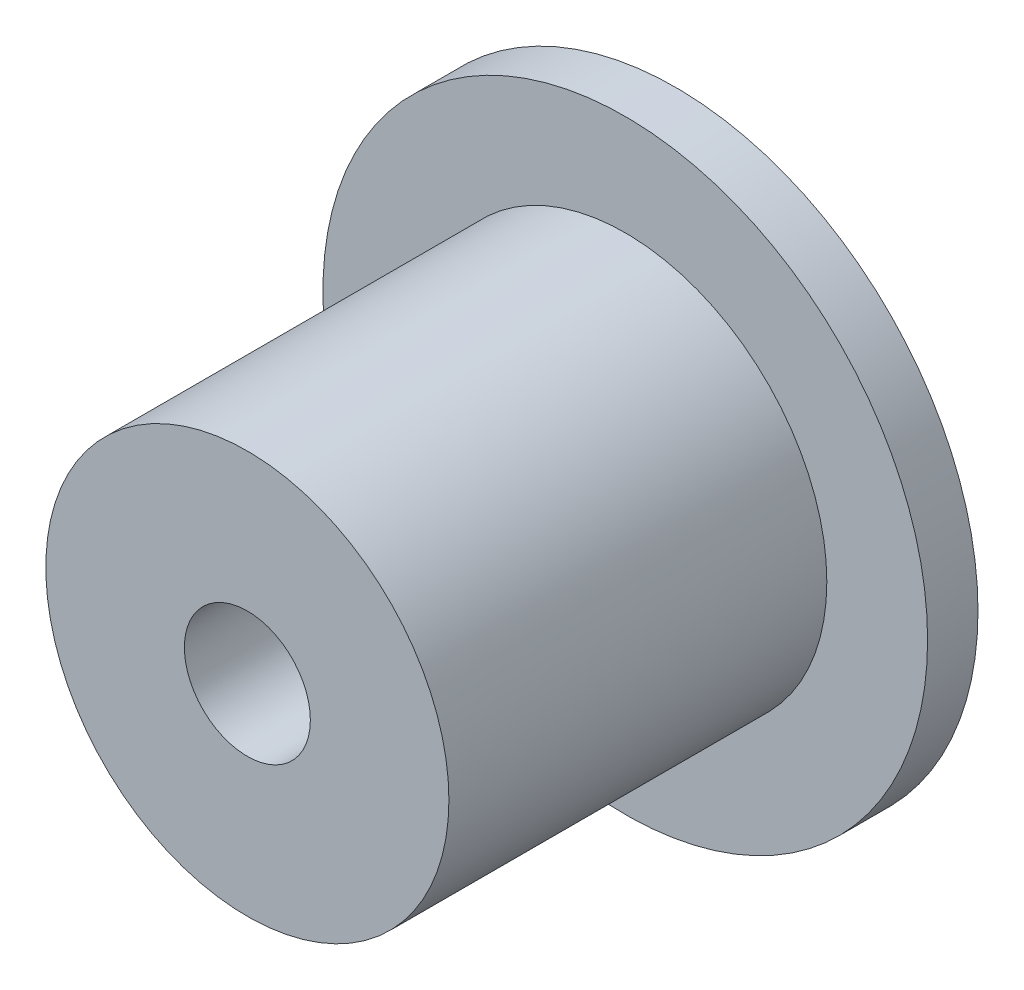
SolidWorks part; units mm, degrees
ref_plane "前视基准面" through (0, 0, 0) normal (0, 0, 1) x (1, 0, 0)
ref_plane "上视基准面" through (0, 0, 0) normal (0, 1, 0) x (1, 0, 0)
ref_plane "右视基准面" through (0, 0, 0) normal (1, 0, 0) x (0, 0, -1)
other "Configuration Table"
sketch "草图1" plane through (0, 0, 0) normal (0, 0, 1) x (1, 0, 0)
  circle A0 centre (0, 0) radius 4
  circle A1 centre (0, 0) radius 1.25
  point P0 (0, 0)
  dimension "D1" = 2.5
  dimension "D2" = 8
extrude "凸台-拉伸1" add sketch "草图1" along normal blind 7.5
sketch "草图2" plane through (0, 0, 0) normal (0, 0, 1) x (1, 0, 0)
  circle A0 centre (0, 0) radius 6
  circle A1 centre (0, 0) radius 1.25
  point P0 (0, 0)
  dimension "D1" = 2.5
  dimension "D2" = 12
extrude "凸台-拉伸2" add sketch "草图2" against normal blind 1
